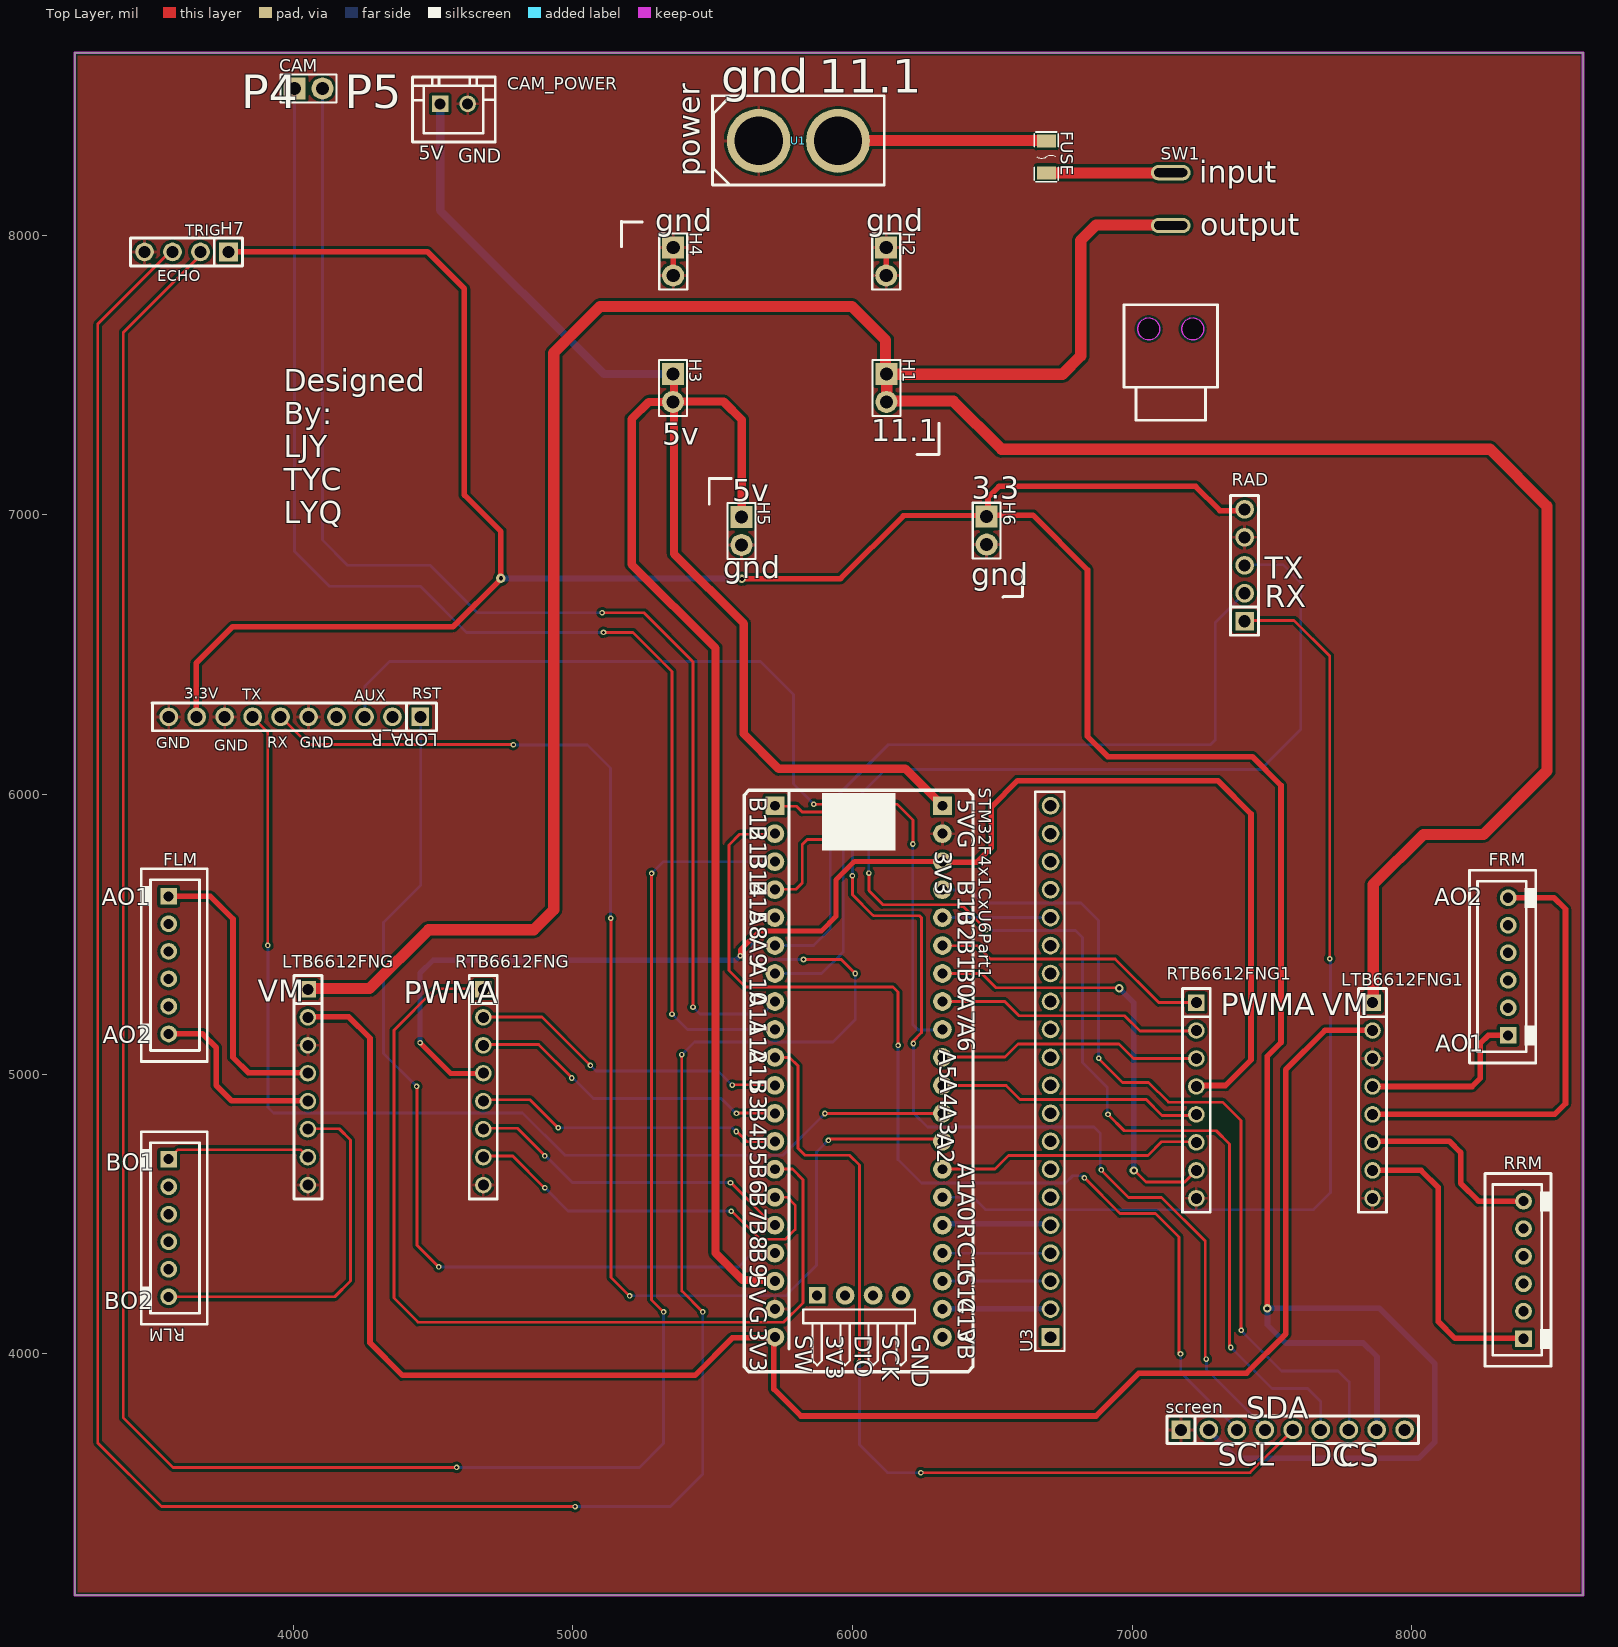
[diagram p0: Top Layer view]
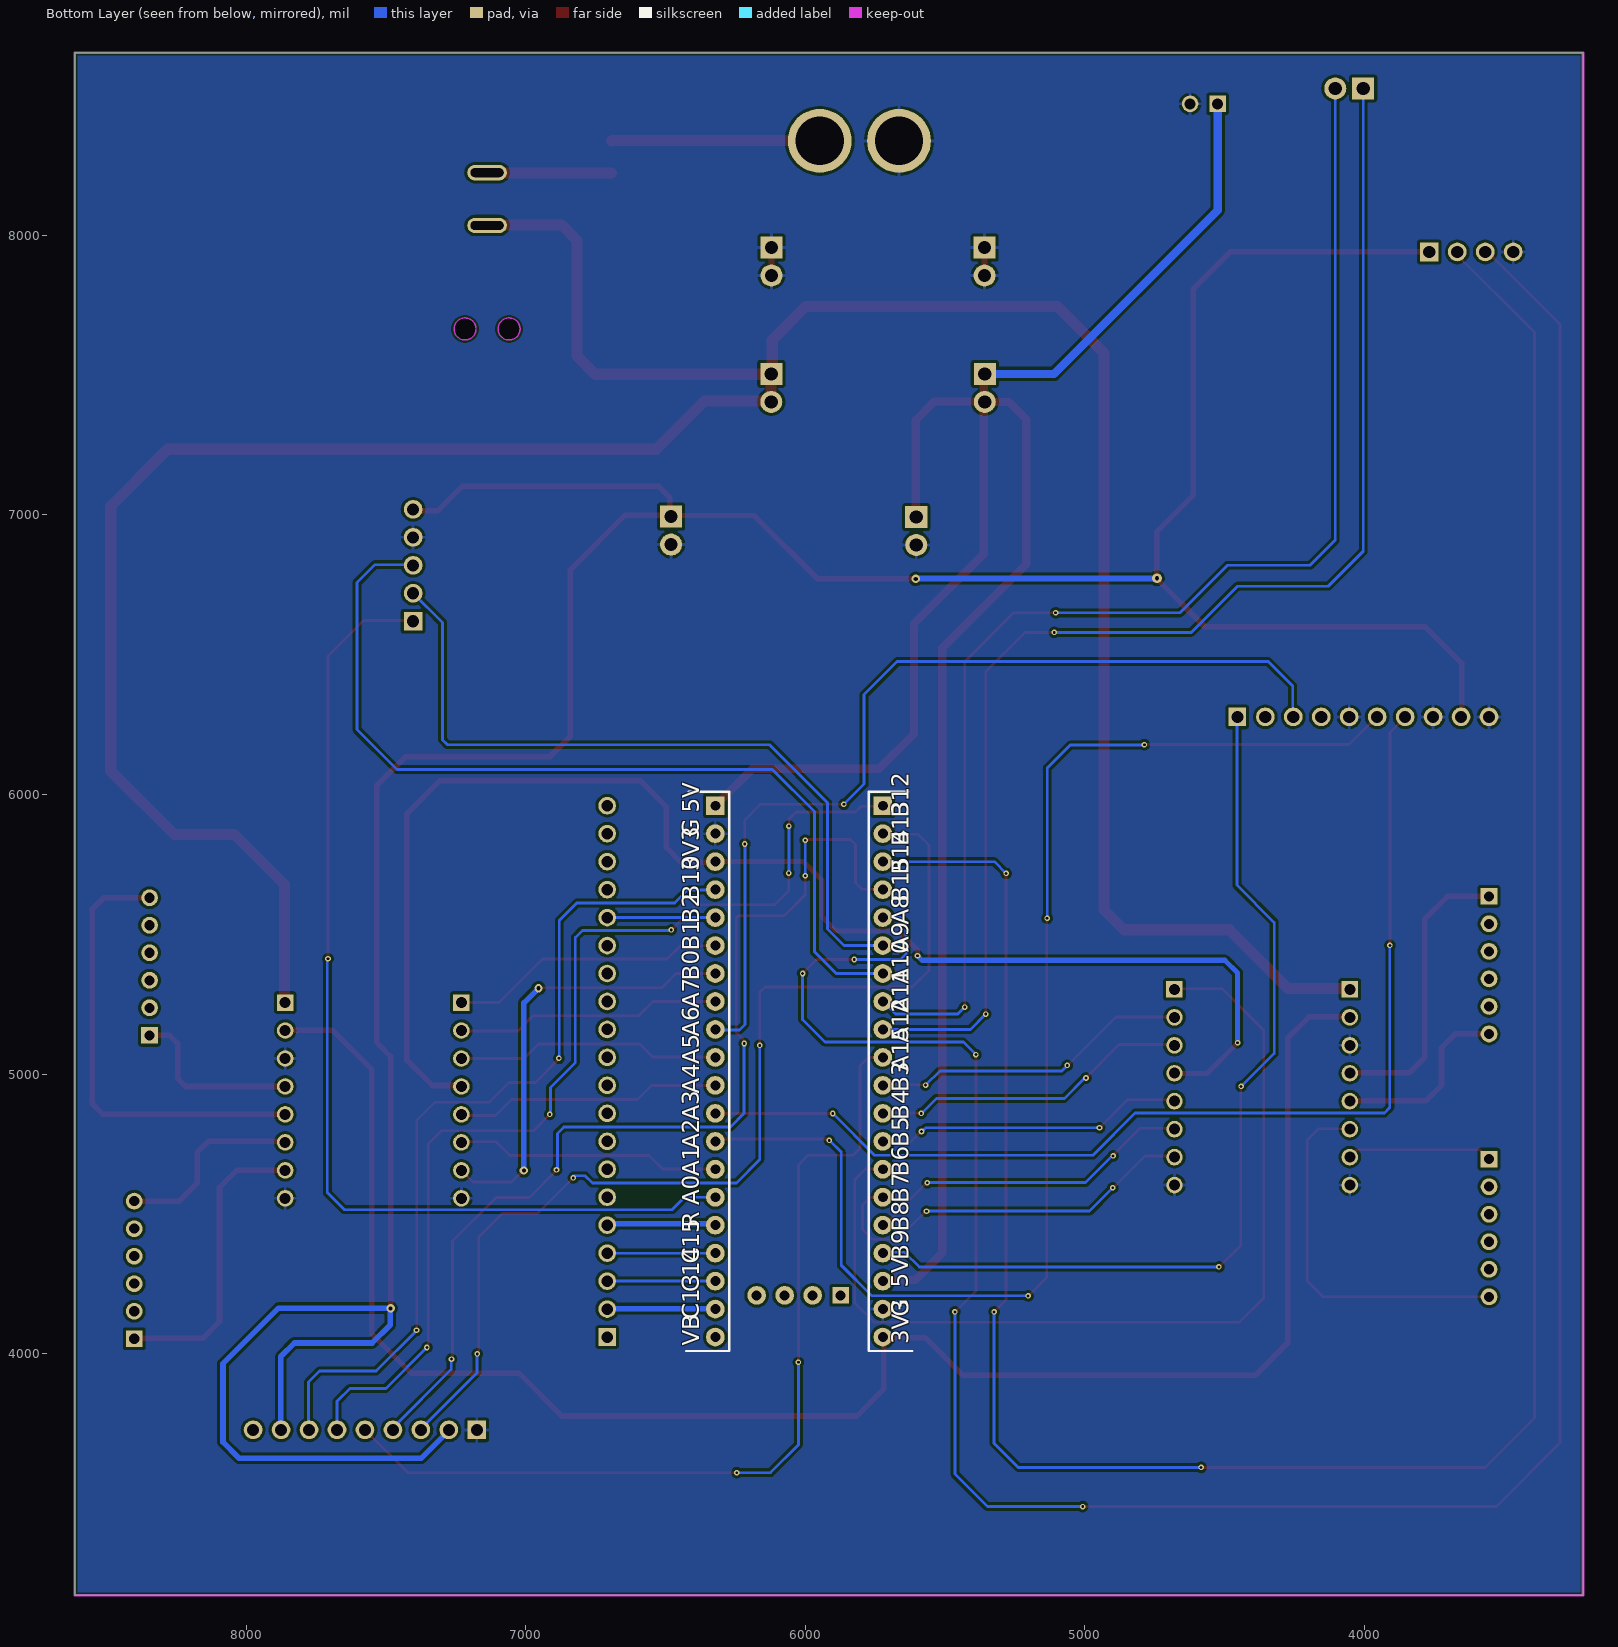
[diagram p1: Bottom Layer view, seen from below]
# Altium PCB MISC51978.pcbdoc
Units mil, origin at the board's own origin, x right, y up, seen from the top; angles counter-clockwise.
Board outline 5393.7 x 5516.21 mil, 2 copper layers (Top Layer, Bottom Layer), stack 62.206 mil thick; 25 components, 49 nets, 170 pads, 57 vias.

## Layer stack, top to bottom
Top Solder Mask Layer: solder mask 0.394, Dk 3.3
Top Layer: signal copper 1.379
Dielectric1: surface 59.449, FR4, Dk 4.5
Bottom Layer: signal copper 1.378
Bottom Solder Mask Layer: solder mask 0.394, Dk 3.3

## Board outline
3219.03,8652.78 3219.03,3136.57 8612.73,3136.57 8612.73,8652.78

## Design rules (kind name [scope] priority, off if disabled: settings)
BoardOutlineClearance copperThickness2oz_1 [All] p2 off: genericclearance=7.99 ignorepadtopadclearanceinfootprint=FALSE except(0: Arc-SplitContinuation Track-SplitContinuation SMDPad-SplitContinuation THPad-SplitContinuation Via-SplitContinuation Fill-SplitContinuation Region-SplitContinuation Poly-SplitContinuation Text-SplitContinuation Hole-SplitContinuation; 5.98: Arc-CutoutEdge SMDPad-CutoutEdge THPad-CutoutEdge Via-CutoutEdge Fill-CutoutEdge Region-CutoutEdge Text-CutoutEdge; 6.93: Hole-OutlineEdge Hole-CutoutEdge; 10: Poly-OutlineEdge Poly-CutoutEdge; 11.81: Arc-OutlineEdge Track-OutlineEdge SMDPad-OutlineEdge THPad-OutlineEdge Via-OutlineEdge Fill-OutlineEdge Region-OutlineEdge Text-OutlineEdge Track-CutoutEdge)
BoardOutlineClearance copperThickness1oz_1 [All] p4: genericclearance=6 ignorepadtopadclearanceinfootprint=FALSE except(0: Arc-SplitContinuation Track-SplitContinuation SMDPad-SplitContinuation THPad-SplitContinuation Via-SplitContinuation Fill-SplitContinuation Region-SplitContinuation Poly-SplitContinuation Text-SplitContinuation Hole-SplitContinuation; 6: Arc-CutoutEdge Track-CutoutEdge SMDPad-CutoutEdge THPad-CutoutEdge Via-CutoutEdge Text-CutoutEdge; 6.93: Hole-OutlineEdge Hole-CutoutEdge; 10: Poly-OutlineEdge Poly-CutoutEdge; 11.8: Arc-OutlineEdge Track-OutlineEdge SMDPad-OutlineEdge THPad-OutlineEdge Via-OutlineEdge Fill-OutlineEdge Region-OutlineEdge Text-OutlineEdge Fill-CutoutEdge Region-CutoutEdge)
Clearance copperThickness2oz [All] p1 off: gap=7.99 ignorepadtopadclearanceinfootprint=FALSE except(5.98: SMDPad-Track SMDPad-SMDPad THPad-Track SMDPad-THPad THPad-THPad Track-Via SMDPad-Via THPad-Via Via-Via Fill-Track Region-Track Fill-SMDPad Region-SMDPad Fill-THPad Region-THPad Fill-Via Region-Via Fill-Fill Fill-Region Region-Region Arc-Track Arc-SMDPad Arc-THPad Arc-Via Fill-Arc Region-Arc Arc-Arc Text-Track SMDPad-Text Text-THPad Text-Via Fill-Text Region-Text Arc-Text Text-Text; 6.93: Hole-Track Hole-SMDPad Hole-THPad Hole-Via Fill-Hole Region-Hole Hole-Arc Hole-Text; 10: Poly-Track Poly-SMDPad Poly-THPad Poly-Via Poly-Fill Poly-Region Poly-Poly Poly-Arc Poly-Text Poly-Hole)
Clearance copperThickness1oz [All] p3: gap=6 ignorepadtopadclearanceinfootprint=FALSE except(5.98: SMDPad-Track SMDPad-SMDPad THPad-Track SMDPad-THPad THPad-THPad Track-Via SMDPad-Via THPad-Via Via-Via Fill-SMDPad Region-SMDPad Fill-THPad Region-THPad Fill-Via Region-Via Fill-Fill Fill-Region Region-Region; 6.93: Hole-Track Hole-SMDPad Hole-THPad Hole-Via Fill-Hole Region-Hole Hole-Arc Hole-Text; 10: Poly-Track Poly-SMDPad Poly-THPad Poly-Via Poly-Fill Poly-Region Poly-Poly Poly-Arc Poly-Text Poly-Hole; 11.8: Fill-Track Region-Track)
DiffPairsRouting differentialPair [All] p1: maxlimit=6 minlimit=6 mostfreqgap=6 toplayer_minwidth=5 toplayer_prefwidth=10 toplayer_maxwidth=100 toplayer_mingap=6 toplayer_prefgap=6 toplayer_maxgap=6 bottomlayer_minwidth=5 bottomlayer_prefwidth=10 bottomlayer_maxwidth=100 bottomlayer_mingap=6 bottomlayer_prefgap=6 bottomlayer_maxgap=6 maxuncoupledlength=10
HoleToHoleClearance otherClearance [All] p1: gap=11.81 allowstackedmicrovias=TRUE
Length netLength [All] p1: minlimit=0 maxlimit=0
MatchedLengths netLengthTolerance [All] p1: tolerance=1000
PasteMaskExpansion pasteMaskExpansion [All] p1: expansion=0
PlaneConnect innerPlane [All] p1: planeconnectstyle=Relief reliefexpansion=20 reliefentries=4 reliefconductorwidth=10 reliefairgap=10
PolygonConnect "copperRegion_Top Layer" [(InNet('GND')) And OnLayer('Top Layer')] p1: connectstyle=Relief reliefconductorwidth=10 reliefentries=4 polygonreliefangle="90 Angle" airgapwidth=10 via.connectstyle=Relief via.reliefconductorwidth=10 via.reliefentries=4 via.polygonreliefangle="90 Angle" via.airgapwidth=10
PolygonConnect "copperRegion_Bottom Layer" [(InNet('GND')) And OnLayer('Bottom Layer')] p2: connectstyle=Relief reliefconductorwidth=10 reliefentries=4 polygonreliefangle="90 Angle" airgapwidth=10 via.connectstyle=Relief via.reliefconductorwidth=10 via.reliefentries=4 via.polygonreliefangle="90 Angle" via.airgapwidth=10
PolygonConnect copperRegion [(InNet('GND'))] p3: connectstyle=Direct reliefconductorwidth=10 reliefentries=4 polygonreliefangle="90 Angle" airgapwidth=10 via.connectstyle=Relief via.reliefconductorwidth=10 via.reliefentries=4 via.polygonreliefangle="90 Angle" via.airgapwidth=10
RoutingVias viaSize [All] p1: holewidth=10 width=20 viastyle="Through Hole" minholewidth=9 minwidth=19.68 maxholewidth=248.03 maxwidth=393.7
SolderMaskExpansion solderMaskExpansion [IsVia] p1: expansion=-1000 istentingtop=TRUE
SolderMaskExpansion solderMaskExpansion [All] p2: expansion=2 istentingtop=FALSE
Width copperThickness2oz_2 [All] p1 off: maxlimit=100 minlimit=8 preferedwidth=10
Width copperThickness1oz_2 [All] p2: maxlimit=10 minlimit=10 preferedwidth=10 toplayer_minwidth=5 toplayer_maxwidth=100 toplayer_prefwidth=10 bottomlayer_minwidth=5 bottomlayer_maxwidth=100 bottomlayer_prefwidth=10

## Components (designator, comment, footprint, x,y, rotation, side; value= is the part's Value field where it differs from the comment)
CAM "PZ254V-11-02P" HDR-TH_2P-P2.54-V-M 4055,8525 r0 top
CAM_POWER "HX-XH2.54-2PZZ" CONN-TH_2P-P2.50_HX-2.54MM-2P-ZZ-MS 4575,8470 r0 top
FLM "HX-XH2.54-6PZZ" CONN-TH_6P-P2.50_BX-XH2.54-6PZZ 3555,5390 r270 top
FRM "HX-XH2.54-6PZZ" CONN-TH_6P-P2.50_BX-XH2.54-6PZZ 8345,5385 r90 top
FUSE "" F1206 6693.35,8280.21 r270 top
H1 "PZ254V-11-02P" HDR-TH_2P-P2.54-V-M 6121.83,7454.08 r270 top
H2 "PZ254V-11-02P" HDR-TH_2P-P2.54-V-M 6120.91,7906.02 r270 top
H3 "PZ254V-11-02P" HDR-TH_2P-P2.54-V-M 5358.22,7454 r270 top
H4 "PZ254V-11-02P" HDR-TH_2P-P2.54-V-M 5359.02,7905.96 r270 top
H5 "PZ254V-11-02P" HDR-TH_2P-P2.54-V-M 5603.37,6942.34 r270 top
H6 "PZ254V-11-02P" HDR-TH_2P-P2.54-V-M 6480.05,6943.82 r270 top
H7 "PZ254V-11-04P" HDR-TH_4P-P2.54-V-M 3618.69,7940.45 r180 top
LORA_R "PZ254V-11-10P" HDR-TH_10P-P2.54-V-M 4005.16,6277.81 r180 top
LTB6612FNG "PZ254V-11-08P" HDR-TH_8P-P2.54-V-M 4052.95,4953.4 r270 top
LTB6612FNG1 "PZ254V-11-08P" HDR-TH_8P-P2.54-V-M 7860.02,4906.07 r270 top
RAD "PZ254V-11-05P" HDR-TH_5P-P2.54-V-M 7402.6,6819.77 r90 top
RLM "HX-XH2.54-6PZZ" CONN-TH_6P-P2.50_BX-XH2.54-6PZZ 3555,4450 r270 top
RRM "HX-XH2.54-6PZZ" CONN-TH_6P-P2.50_BX-XH2.54-6PZZ 8400,4300 r90 top
RTB6612FNG "PZ254V-11-08P" HDR-TH_8P-P2.54-V-M 4680.06,4953.4 r270 top
RTB6612FNG1 "PZ254V-11-08P" HDR-TH_8P-P2.54-V-M 7230.02,4906.07 r270 top
screen "PZ254V-11-09P" HDR-TH_9P-P2.54-V-M 7574.85,3728.09 r0 top
STM32F4x1CxU6Part1 "STM32F4x1CxU6 WeActStudio" "STM32F4x1CxU6 WeActStudio" 5975,5245 r270 top
SW1 "HX KCD11-BL" SW-TH_KCD11-BL 7138.26,8129.56 r0 top
U1 "XT60-M." CONN-TH_XT60 5806.73,8337.63 r0 top
U3 "ZX-PZ2.54-1-20PZZ" HDR-TH_20P-P2.54-V-M 6708.51,5010 r90 top

## Footprints (in the part's own frame and the unit in brackets; to place one, negate y for a bottom-side part, rotate by r counter-clockwise, add the part's x,y. Pads: shape width x height; smd on the part's side, far side on the other; paste and mask are expansions set on the pad)
CONN-TH_2P-P2.50_HX-2.54MM-2P-ZZ-MS [mm]
  rect 1.5x1.5 hole 1: 1(-1.25,0)
  round 1.5 hole 1: 2(1.25,0)
  silkscreen extent -3.75,-3.46 3.75,2.44
CONN-TH_6P-P2.50_BX-XH2.54-6PZZ [mil]
  rect 60x60 hole 36: 1(-246.07,0)
  round 60 hole 36: 2(-147.65,0) 3(-49.22,0) 4(49.2,0) 5(147.63,0) 6(246.06,0)
  silkscreen extent -344,-100 344,138
CONN-TH_XT60 [mm]
  round 5.8 hole 4.4 paste+0 mask+0.05: 1(-3.6,0) 2(3.6,0)
  silkscreen extent -7.8,-4 7.8,4.1
F1206 [mm]
  rect 1.19x1.728 smd: 1(-1.445,0) 2(1.445,0)
  silkscreen extent -2.27,-1.09 2.27,1.09
HDR-TH_2P-P2.54-V-M [mm]
  rect 2x2 hole 1.2: 1(-1.27,0)
  round 2 hole 1.2: 2(1.27,0)
  silkscreen extent -2.54,-1.27 2.54,1.27
HDR-TH_4P-P2.54-V-M [mm]
  rect 1.7x1.7 hole 1.1: 1(-3.81,0)
  round 1.7 hole 1.1: 2(-1.27,0) 3(1.27,0) 4(3.81,0)
  silkscreen extent -5.08,-1.27 5.08,1.27
HDR-TH_5P-P2.54-V-M [mm]
  rect 1.7x1.7 hole 1.1: 1(-5.08,0)
  round 1.7 hole 1.1: 2(-2.54,0) 3(0,0) 4(2.54,0) 5(5.08,0)
  silkscreen extent -6.35,-1.27 6.35,1.27
HDR-TH_8P-P2.54-V-M [mm]
  rect 1.5x1.5 hole 1: 1(-8.89,0)
  round 1.5 hole 1: 2(-6.35,0) 3(-3.81,0) 4(-1.27,0) 5(1.27,0) 6(3.81,0) 7(6.35,0) 8(8.89,0)
  silkscreen extent -10.16,-1.27 10.16,1.27
HDR-TH_9P-P2.54-V-M [mm]
  rect 1.7x1.7 hole 1.1: 1(-10.16,0)
  round 1.7 hole 1.1: 2(-7.62,0) 3(-5.08,0) 4(-2.54,0) 5(0,0) 6(2.54,0) 7(5.08,0) 8(7.62,0) 9(10.16,0)
  silkscreen extent -11.43,-1.25 11.43,1.25
HDR-TH_10P-P2.54-V-M [mm]
  rect 1.575x1.7 hole 1.1: 1(-11.43,0)
  round 1.7 hole 1.1: 2(-8.89,0) 3(-6.35,0) 4(-3.81,0) 5(-1.27,0) 6(1.27,0) 7(3.81,0) 8(6.35,0) 9(8.89,0) 10(11.43,0)
  silkscreen extent -12.9,-1.27 12.95,1.27
HDR-TH_20P-P2.54-V-M [mm]
  rect 1.6x1.6 hole 1.05: 1(-24.13,0)
  round 1.6 hole 1.05: 2(-21.59,0) 3(-19.05,0) 4(-16.51,0) 5(-13.97,0) 6(-11.43,0) 7(-8.89,0) 8(-6.35,0) 9(-3.81,0) 10(-1.27,0) 11(1.27,0) 12(3.81,0) 13(6.35,0) 14(8.89,0) 15(11.43,0) 16(13.97,0) 17(16.51,0) 18(19.05,0) 19(21.59,0) 20(24.13,0)
  silkscreen extent -25.4,-1.27 25.4,1.4
"STM32F4x1CxU6 WeActStudio" [mm]
  rect 1.7x1.7 hole 0.9: 1(-18.161,-6.401) 40(-18.161,8.814)
  round 1.7 hole 0.9: 2(-15.621,-6.401) 3(-13.081,-6.401) 4(-10.541,-6.401) 5(-8.001,-6.401) 6(-5.461,-6.401) 7(-2.921,-6.401) 8(-0.381,-6.401) 9(2.159,-6.401) 10(4.699,-6.401) 11(7.239,-6.401) 12(9.779,-6.401) 13(12.319,-6.401) 14(14.859,-6.401) 15(17.399,-6.401) 16(19.939,-6.401) 17(22.479,-6.401) 18(25.019,-6.401) 19(27.559,-6.401) 20(30.099,-6.401) 21(30.099,8.814) 22(27.559,8.814) 23(25.019,8.814) 24(22.479,8.814) 25(19.939,8.814) 26(17.399,8.814) 27(14.859,8.814) 28(12.319,8.814) 29(9.779,8.814) 30(7.239,8.814) 31(4.699,8.814) 32(2.159,8.814) 33(-0.381,8.814) 34(-2.921,8.814) 35(-5.461,8.814) 36(-8.001,8.814) 37(-10.541,8.814) 38(-13.081,8.814) 39(-15.621,8.814) 42(26.314,-0.025) 43(26.314,2.515) 44(26.314,5.055)
  rect 1.5x1.5 hole 0.9: 41(26.314,-2.565)
  silkscreen extent -19.56,-9.19 33.25,11.58
SW-TH_KCD11-BL [mm]
  oval 3.6x1.4 hole 0.8 slot 3 at 0 deg paste+0 mask+0.05: 1(0,2.4) 2(0,-2.4)
  Board Outline Layer circle w0.003: c-2,-11.8 r1
  Board Outline Layer circle w0.003: c2,-11.8 r1
  Board Outline Layer region: -1,-11.8 -1.099,-12.234 -1.377,-12.582 -1.777,-12.775 -2.223,-12.775 -2.623,-12.582 -2.901,-12.234 -3,-11.8 -3,-11.8 -2.901,-11.366 -2.623,-11.018 -2.223,-10.825 -1.777,-10.825 -1.377,-11.018 -1.099,-11.366 -1,-11.8
  Board Outline Layer region: -1,-11.8 -1.009,-11.936 -1.037,-12.07 -1.083,-12.198 -1.146,-12.319 -1.224,-12.431 -1.317,-12.531 -1.423,-12.617 -1.54,-12.688 -1.665,-12.742 -1.797,-12.779 -1.932,-12.798 -2.068,-12.798 -2.203,-12.779 -2.335,-12.742 -2.46,-12.688 -2.577,-12.617 -2.683,-12.531 -2.776,-12.431 -2.854,-12.319 -2.917,-12.198 -2.963,-12.07 -2.991,-11.936 -3,-11.8 -2.991,-11.664 -2.963,-11.53 -2.917,-11.401 -2.854,-11.28 -2.776,-11.169 -2.683,-11.069 -2.577,-10.983 -2.46,-10.912 -2.335,-10.858 -2.203,-10.821 -2.068,-10.802 -1.932,-10.802 -1.797,-10.821 -1.665,-10.858 -1.54,-10.912 -1.423,-10.983 -1.317,-11.069 -1.224,-11.169 -1.146,-11.28 -1.083,-11.401 -1.037,-11.53 -1.009,-11.664
  Board Outline Layer region: 3,-11.8 2.901,-12.234 2.623,-12.582 2.223,-12.775 1.777,-12.775 1.377,-12.582 1.099,-12.234 1,-11.8 1,-11.8 1.099,-11.366 1.377,-11.018 1.777,-10.825 2.223,-10.825 2.623,-11.018 2.901,-11.366 3,-11.8
  Board Outline Layer region: 3,-11.8 2.991,-11.936 2.963,-12.07 2.917,-12.198 2.854,-12.319 2.776,-12.431 2.683,-12.531 2.577,-12.617 2.46,-12.688 2.335,-12.742 2.203,-12.779 2.068,-12.798 1.932,-12.798 1.797,-12.779 1.665,-12.742 1.54,-12.688 1.423,-12.617 1.317,-12.531 1.224,-12.431 1.146,-12.319 1.083,-12.198 1.037,-12.07 1.009,-11.936 1,-11.8 1.009,-11.664 1.037,-11.53 1.083,-11.401 1.146,-11.28 1.224,-11.169 1.317,-11.069 1.423,-10.983 1.54,-10.912 1.665,-10.858 1.797,-10.821 1.932,-10.802 2.068,-10.802 2.203,-10.821 2.335,-10.858 2.46,-10.912 2.577,-10.983 2.683,-11.069 2.776,-11.169 2.854,-11.28 2.917,-11.401 2.963,-11.53 2.991,-11.664
  Multi-Layer board cut-out: -1,-11.8 -1.099,-12.234 -1.377,-12.582 -1.777,-12.775 -2.223,-12.775 -2.623,-12.582 -2.901,-12.234 -3,-11.8 -3,-11.8 -2.901,-11.366 -2.623,-11.018 -2.223,-10.825 -1.777,-10.825 -1.377,-11.018 -1.099,-11.366 -1,-11.8
  Multi-Layer board cut-out: 3,-11.8 2.901,-12.234 2.623,-12.582 2.223,-12.775 1.777,-12.775 1.377,-12.582 1.099,-12.234 1,-11.8 1,-11.8 1.099,-11.366 1.377,-11.018 1.777,-10.825 2.223,-10.825 2.623,-11.018 2.901,-11.366 3,-11.8
  silkscreen extent -4.25,-20.1 4.25,-9.6

## Via types
v1: diameter 20, hole 10, Top Layer to Bottom Layer, 52 vias
v2: diameter 30, hole 15, Top Layer to Bottom Layer, 4 vias
v3: diameter 35, hole 15, Top Layer to Bottom Layer, 1 vias

## Nets (pads, with @x,y where several pads share a name; then routed paths per layer and width w, separated by ;. In a path a pad name is that pad's centre, name@x,y a point inside that pad or via, vN(x,y) a via of type N, cw(c..) or ccw(c..) an arc to the next point about the centre after c; other vN are vias at no path point)
CAM_P4: CAM.1 STM32F4x1CxU6Part1.9 | length 4798.9
  Top Layer w10: v1(5110,6580) 5215,6580 5355,6440 v1(5355,5215)
  Bottom Layer w10: CAM.1 4005,6870 4130,6745 4455,6745 4620,6580 v1(5110,6580) ; v1(5355,5215) 5410,5160 STM32F4x1CxU6Part1.9
CAM_P5: CAM.2 STM32F4x1CxU6Part1.8 | length 4677.2
  Top Layer w10: v1(5105,6650) 5255,6650 5430,6475 v1(5430,5240)
  Bottom Layer w10: CAM.2 4105,6910 4195,6820 4490,6820 4660,6650 v1(5105,6650) ; v1(5430,5240) 5455,5215 5678,5215 STM32F4x1CxU6Part1.8
GND: CAM_POWER.2 H2.1 H2.2 H4.1 H4.2 H5.2 H6.2 H7.4 LORA_R.5 LORA_R.8 LORA_R.10 LTB6612FNG1.3 LTB6612FNG1.8 LTB6612FNG.3 LTB6612FNG.8 RAD.4 RTB6612FNG1.8 RTB6612FNG.8 screen.1 STM32F4x1CxU6Part1.19 STM32F4x1CxU6Part1.39 U1.1 | length 201.1
  Top Layer w20: H4.2@5359.4,7854.66 H4.1@5359.4,7955.86 ; H2.2@6121.01,7857.25 H2.1@6121.01,7957.15
HC_ECHO: H7.3 STM32F4x1CxU6Part1.5 | length 9646.4
  Top Layer w10: H7.3@3563.74,7944.74 3301,7682.01 3301,3681.84 3529.03,3453.82 v1(5008.21,3453.82) ; v1(5390,5070) 5390,4225 v1(5465,4150) ; v1(5825,5410) 5960,5410 v1(6010,5360)
  Bottom Layer w10: v1(5008.21,3453.82) 5348.82,3453.82 5465,3570 v1(5465,4150) ; v1(5390,5070) 5435,5115 5930,5115 6010,5195 v1(6010,5360) ; STM32F4x1CxU6Part1.5 5660,5560 5640,5540 5640,5430 5660,5410 v1(5825,5410)
HC_TRIG: H7.2 STM32F4x1CxU6Part1.3 | length 8841.6
  Top Layer w10: H7.2@3678.57,7938.78 3392.84,7653.06 3392.84,3771.13 3570.11,3593.86 v1(4584.69,3593.86) ; v1(5281.96,5718.04) 5281.96,4193.04 v1(5325,4150)
  Bottom Layer w10: v1(4584.69,3593.86) 5238.86,3593.86 5325,3680 v1(5325,4150) ; v1(5281.96,5718.04) 5323.93,5760 STM32F4x1CxU6Part1.3
L_AIN1: RTB6612FNG.3 STM32F4x1CxU6Part1.12 | length 1136
  Top Layer w10: RTB6612FNG.3@4685.41,5105.65 4878.08,5105.65 v1@4994.85,4988.88 ; v1@5585.63,4861.57 5720.56,4861.57 STM32F4x1CxU6Part1.12@5724.89,4857.24
  Bottom Layer w10: v1@4997.44,4986.13 5000.9,4986.13 5073.56,4913.47 5531.13,4913.47 v1@5583.03,4861.57
  other v1: 5585.63,4859.84 4996.5,4986.28
L_AIN2: RTB6612FNG.2 STM32F4x1CxU6Part1.11 | length 1142.5
  Top Layer w10: RTB6612FNG.2@4676.65,5204.9 4889.46,5204.9 v1(5063.1,5031.26) ; v1@5570.92,4961.91 5720.56,4961.91 STM32F4x1CxU6Part1.11@5721.43,4961.04
  Bottom Layer w10: v1(5063.1,5031.26) 5082.88,5011.48 5518.97,5011.48 v1@5567.89,4962.56
  other v1: 5570.06,4961.04
L_AO1: FLM.1 LTB6612FNG.4 | length 1050
  Top Layer w20: FLM.1 3703.93,5636.06 3785,5555 3785,5060 3840,5005 4051.34,5005 LTB6612FNG.4
L_AO2: FLM.6 LTB6612FNG.5 | length 676.7
  Top Layer w20: FLM.6 3676.07,5143.94 3725,5095 3725,4960 3780,4905 4051.34,4905 LTB6612FNG.5
L_BIN1: RTB6612FNG.5 STM32F4x1CxU6Part1.13 | length 1096.1
  Top Layer w10: RTB6612FNG.5@4683.38,4908.76 4847.4,4908.76 v1(4948.06,4808.1) ; v1@5586.49,4794.97 5622.82,4758.64 STM32F4x1CxU6Part1.13@5721.43,4758.64
  Bottom Layer w10: v1(4948.06,4808.1) 4948.77,4808.81 5569.19,4808.81 v1@5582.17,4795.83
  other v1: 5584.76,4794.97
L_BIN2: RTB6612FNG.6 STM32F4x1CxU6Part1.16 | length 1169.6
  Top Layer w10: RTB6612FNG.6@4686.3,4806.58 4803.07,4806.58 v1@4899.41,4710.25 ; v1@5566.6,4610.73 5719.7,4457.63 STM32F4x1CxU6Part1.16@5722.29,4457.63
  Bottom Layer w10: v1@4901.43,4709.33 4998.31,4612.46 v1@5558.81,4612.46
  other v1: 5564,4611.59 4899.62,4707.76
L_BO1: LTB6612FNG.7 RLM.1 | length 523
  Top Layer w10: RLM.1 3588.93,4730 4026.34,4730 LTB6612FNG.7
L_BO2: LTB6612FNG.6 RLM.6 | length 1347.5
  Top Layer w10: RLM.6 4148.94,4203.94 4205,4260 4205,4765 4165,4805 4054.55,4805 LTB6612FNG.6
L_PWMA: RTB6612FNG.1 STM32F4x1CxU6Part1.14 | length 3417
  Top Layer w10: RTB6612FNG.1@4681.84,5305.78 4509.6,5305.78 4360.71,5156.9 4360.71,4199.37 4446.94,4113.15 5754.57,4113.15 5823.28,4181.85 5823.28,4622.67 5785.33,4660.62 STM32F4x1CxU6Part1.14@5729.86,4660.62
L_PWMB: RTB6612FNG.7 STM32F4x1CxU6Part1.15 | length 1410.4
  Top Layer w10: RTB6612FNG.7@4686.3,4707.33 4785.55,4707.33 v1@4899.41,4593.47 ; v1@5570.06,4509.52 5669.53,4410.05 5761.22,4410.05 5795.38,4444.22 5795.38,4531.58 5767.27,4559.69 STM32F4x1CxU6Part1.15@5725.75,4559.69
  Bottom Layer w10: v1@4899.7,4594.29 4983.6,4510.39 v1@5565.73,4510.39
  other v1: 5566.6,4509.52 4900.49,4593.58
LORA_AUX: LORA_R.3 STM32F4x1CxU6Part1.32 | length 3357.7
  Top Layer w10: v1@5864.14,5965.65 6159.96,5965.65 6216.4,5909.21 v1@6216.4,5823.57
  Bottom Layer w10: LORA_R.3@4257.2,6287.4 4257.2,6388.11 4344.78,6475.69 5671.6,6475.69 5789.83,6357.46 5789.83,6037.8 v1@5859.89,5967.74 ; v1@6215.88,5823.72 6215.88,5177.58 6235.34,5158.12 6317.08,5158.12 STM32F4x1CxU6Part1.32@6319.67,5160.71
  other v1: 6216.4,5823.24 5862.1,5965.14
LORA_RST: LORA_R.1 STM32F4x1CxU6Part1.17 | length 3330.7
  Top Layer w10: v1@4442.72,4957.37 4442.72,4388.26 v1@4520.57,4310.41
  Bottom Layer w10: v1@4441.94,4955.84 4323.51,5074.27 4323.51,5543.04 4456.74,5676.27 LORA_R.1@4456.74,6278.27 ; v1@4521.55,4310.29 5592.31,4310.29 5644.95,4362.92 5722.25,4362.92 STM32F4x1CxU6Part1.17@5723.9,4361.28
  other v1: 4520.94,4310.9 4441.62,4956.27
LORA_RX: LORA_R.6 STM32F4x1CxU6Part1.28 | length 4743.9
  Top Layer w10: LORA_R.6@3956.64,6277.74 4055.6,6178.78 v1@4787.81,6178.78 ; v1@5136.53,5557.82 5136.53,4273.22 v1@5202.32,4207.43 ; v1@5917.14,4768.52 6311.89,4768.52 STM32F4x1CxU6Part1.28@6316.83,4763.59
  Bottom Layer w10: v1@4791.91,6176.68 5052.67,6176.68 5134.94,6094.41 ; v1@5134.94,5558.43 5134.94,6090.51 ; 5134.94,6094.63 5134.94,6094.41 ; v1@5205.24,4207.98 5762.83,4207.98 5871.39,4316.54 5871.39,4721.16 v1@5913.33,4763.1 ; 5134.94,6090.51 5135.13,6090.32 5134.94,6094.03 ; 5134.94,6090.51 5134.94,6094.03 ; 5134.94,6094.03 5134.94,6094.41
  other v1: 5203.42,4207.07 5914.22,4763.38 5135.61,5557.27 4787.63,6178.32
LORA_TX: LORA_R.7 STM32F4x1CxU6Part1.29 | length 3959.6
  Top Layer w10: LORA_R.7@3858.05,6273.73 3909.56,6222.22 v1(3909.56,5460.43) ; v1@5902.23,4859.72 6321.84,4859.72 STM32F4x1CxU6Part1.29@6322.82,4860.69
  Bottom Layer w10: v1(3909.56,5460.43) 3910,5459.98 3910,4880.72 3929.51,4861.2 4820.72,4861.2 4971.77,4710.16 5752.51,4710.16 v1@5901.63,4859.29
  other v1: 5901.75,4859.43
P2_11.1V: FUSE.2 SW1.1 | length 446.7
  Top Layer w40: FUSE.2@6694.06,8223.13 7139.52,8223.13 SW1.1@7140.38,8224
P_3.3V: H6.1 H7.1 LORA_R.9 RAD.5 screen.2 screen.8 | length 12534.8
  Top Layer w10: v3@4742.86,6771.33 v3@4744.8,6771.33
  Top Layer w20: LORA_R.9@3652.99,6280.89 3652.99,6469.67 3783.38,6600.06 4571.59,6600.06 v3@4742.86,6771.33 ; H7.1@3769.76,7940.99 4480.12,7940.99 4612.46,7808.65 4612.46,7071.15 4742.86,6940.76 v3@4742.86,6777.17 ; v2@5607.13,6772.03 5957.44,6772.03 6182.23,6996.82 H6.1@6478.89,6999.18 ; RAD.5@7402.73,7022.87 7395.33,7015.47 7313.91,7015.47 7227.56,7101.82 6524.4,7101.82 6484.93,7062.34 6484.93,6999.21 6645.29,6999.21 6840.88,6803.62 6840.88,6208.09 6913.86,6135.1 7430.58,6135.1 7532.75,6032.93 7532.75,5113.35 7483.12,5063.72 v2@7483.12,4164.58
  Bottom Layer w20: v3@4743.77,6772.6 v2@5603.99,6772.6 ; screen.2@7271.09,3729.38 7374.16,3626.31 8024.41,3626.31 8082.53,3684.43 8082.53,3965.14 7884.05,4163.61 7484.42,4163.61 7484.42,4103.4 7549.01,4038.81 7826.95,4038.81 7875.97,3989.8 7875.97,3730.3 screen.8@7874.82,3729.15
  other v2: 7483.3,4162.5 5604.98,6771.26
  other v3: 4742.88,6773.23
P_5V: CAM_POWER.1 H3.1 H3.2 H5.1 STM32F4x1CxU6Part1.18 STM32F4x1CxU6Part1.40 | length 7796.5
  Top Layer w20: H3.1@5359.72,7505.09 H3.1@5360.79,7505.09
  Top Layer w30: H3.2@5357.13,7403.74 5271.82,7403.74 5210.62,7342.55 5210.62,6823.34 5510.39,6523.58 5510.39,4360.38 5606.73,4264.04 STM32F4x1CxU6Part1.18@5724.96,4264.04 ; H3.1@5359.72,7505.09 H3.1@5359.72,7505.32 ; H3.2@5362.03,7403.74 5362.03,6860.74 5611.63,6611.14 5611.63,6217.04 5736.43,6092.24 6189.65,6092.24 STM32F4x1CxU6Part1.40@6314.45,5967.44 ; H3.2@5362.03,7409.95 H3.1@5362.03,7505.09 ; H3.2@5363.28,7406.97 5540.07,7404.76 5604.94,7339.89 H5.1@5604.94,6993
  Bottom Layer w30: CAM_POWER.1 4525.78,8089.22 5111,7504 H3.1
P_11.1V: FUSE.1 U1.2 | length 744.2
  Top Layer w40: U1.2@5949.91,8338.81 6691.72,8338.81 FUSE.1
PB2: STM32F4x1CxU6Part1.36 U3.16 | length 386.5
  Bottom Layer w10: STM32F4x1CxU6Part1.36 U3.16
PC13: STM32F4x1CxU6Part1.22 U3.2 | length 385.3
  Bottom Layer w20: STM32F4x1CxU6Part1.22@6323.41,4161.87 U3.2@6708.76,4161.87
PC14: STM32F4x1CxU6Part1.23 U3.3 | length 386.5
  Bottom Layer w10: STM32F4x1CxU6Part1.23 U3.3
PC15: STM32F4x1CxU6Part1.24 U3.4 | length 386.5
  Bottom Layer w10: STM32F4x1CxU6Part1.24 U3.4
POWER_11.1V: H1.1 H1.2 LTB6612FNG1.1 LTB6612FNG.1 SW1.2 | length 10649.8
  Top Layer w40: LTB6612FNG.1@4054.52,5306.14 4273.46,5306.14 4483.65,5516.33 4860.24,5516.33 4931.76,5587.85 4931.76,7578.81 5098.16,7745.21 5998.76,7745.21 6118.46,7625.52 H1.1@6118.46,7507.28 ; H1.2@6115.17,7407.51 6360.39,7407.51 6532.91,7235 8280,7235 8484.18,7030.82 8484.18,6085.07 8256.47,5857.37 8041.9,5857.37 7862.37,5677.83 LTB6612FNG1.1@7862.37,5270.59 ; H1.2@6122.96,7408.23 H1.1@6122.96,7501.98 ; H1.1@6123.61,7503.04 6751.58,7503.04 6816.45,7567.92 6816.45,7981.81 6870.94,8036.3 SW1.2@7139.52,8036.3
R_AIN1: RTB6612FNG1.3 STM32F4x1CxU6Part1.31 | length 945.1
  Top Layer w10: STM32F4x1CxU6Part1.31@6324.09,5060.93 6545.52,5060.93 6592.23,5107.64 6953.79,5107.64 7005.69,5055.74 7227.12,5055.74 RTB6612FNG1.3@7227.99,5056.61
R_AIN2: RTB6612FNG1.2 STM32F4x1CxU6Part1.33 | length 950.8
  Top Layer w10: STM32F4x1CxU6Part1.33@6323.23,5259.87 6544.66,5259.87 6595.69,5208.84 6973.69,5208.84 7028.18,5154.35 7225.39,5154.35 RTB6612FNG1.2@7228.85,5157.81
R_AO1: FRM.1 LTB6612FNG1.4 | length 634
  Top Layer w20: LTB6612FNG1.4 8216.07,4956.07 8245,4985 8245,5110 8273.93,5138.94 FRM.1
R_AO2: FRM.6 LTB6612FNG1.5 | length 1623.1
  Top Layer w20: LTB6612FNG1.5 8511.07,4856.07 8550,4895 8550,5590 8508.93,5631.06 FRM.6
R_BIN1: RTB6612FNG1.5 STM32F4x1CxU6Part1.30 | length 953.4
  Top Layer w10: STM32F4x1CxU6Part1.30@6322.36,4959.73 6549.85,4959.73 6600.02,4909.56 7050.67,4909.56 7107.76,4852.47 7228.85,4852.47 RTB6612FNG1.5@7230.58,4854.2
R_BIN2: RTB6612FNG1.6 STM32F4x1CxU6Part1.27 | length 953.7
  Top Layer w10: STM32F4x1CxU6Part1.27@6323.23,4660.88 6510.06,4660.88 6558.5,4709.32 7056.72,4709.32 7105.6,4758.19 RTB6612FNG1.6@7236.64,4758.19
R_BO1: LTB6612FNG1.7 RRM.1 | length 1070.6
  Top Layer w20: LTB6612FNG1.7 8033.93,4656.07 8095,4595 8095,4115 8155,4055 8398.93,4055 RRM.1
R_BO2: LTB6612FNG1.6 RRM.6 | length 694.7
  Top Layer w20: LTB6612FNG1.6 7863.94,4760 8135,4760 8175,4720 8175,4610 8238.93,4546.06 RRM.6
R_PWMA: RTB6612FNG1.1 STM32F4x1CxU6Part1.35 | length 992.9
  Top Layer w10: STM32F4x1CxU6Part1.35@6322.14,5459.03 6447.57,5459.03 6494.27,5412.33 6939.74,5412.33 7095.43,5256.63 RTB6612FNG1.1@7231.23,5256.63
R_PWMB: RTB6612FNG1.7 STM32F4x1CxU6Part1.34 | length 1580.7
  Top Layer w10: STM32F4x1CxU6Part1.34@6321.72,5359.81 6462.43,5359.81 6513.17,5309.06 6953.15,5309.06 v2@6955.46,5306.76 ; v2@7008.88,4656.07 7050.4,4614.55 7188.41,4614.55 RTB6612FNG1.7@7229.93,4656.07
  Bottom Layer w20: v2@6956.49,5305.25 7006.66,5255.08 v2@7006.66,4656.52
  other v2: 7006.58,4655.68 6954.31,5307.33
RAD_OT2: RAD.1 STM32F4x1CxU6Part1.26 | length 3700.7
  Top Layer w10: RAD.1@7407.34,6622.78 7579.43,6622.78 7707.11,6495.11 v1@7707.11,5412.62
  Bottom Layer w10: STM32F4x1CxU6Part1.26@6326.3,4559.82 6431.57,4559.82 6475.82,4515.56 7648.88,4515.56 7709.58,4576.26 v1@7709.58,5415.12
  other v1: 7706.88,5412.62
RAD_RX: RAD.2 STM32F4x1CxU6Part1.6 | length 2722.9
  Bottom Layer w10: STM32F4x1CxU6Part1.6@5713.51,5465.1 5718.45,5460.16 5861.55,5460.16 5920.76,5519.38 5920.76,5970.88 6128.01,6178.12 7280.19,6178.12 7297.46,6195.39 7297.46,6614.63 RAD.2
RAD_TX: RAD.3 STM32F4x1CxU6Part1.7 | length 3282.1
  Bottom Layer w10: STM32F4x1CxU6Part1.7 5889.68,5360 5967.64,5437.96 5967.64,5938.8 6118.14,6089.3 7460.3,6089.3 7603.4,6232.4 7603.4,6757.92 7539.25,6822.06 RAD.3@7408.49,6822.06
RST: STM32F4x1CxU6Part1.25 U3.5 | length 392.4
  Bottom Layer w20: STM32F4x1CxU6Part1.25@6320.5,4465.48 6708.76,4465.48 U3.5@6711.68,4462.56
S1_3.3V: LTB6612FNG1.2 LTB6612FNG.2 STM32F4x1CxU6Part1.20 | length 6374.7
  Top Layer w20: LTB6612FNG.2@4055.87,5204.69 4198.91,5204.69 4274.81,5128.79 4274.81,4039.46 4391.15,3923.12 5436.69,3923.12 5570.98,4057.41 STM32F4x1CxU6Part1.20@5719.49,4057.41 ; STM32F4x1CxU6Part1.20@5719.49,4062.19 STM32F4x1CxU6Part1.20@5719.49,4057.41 ; STM32F4x1CxU6Part1.20@5728.62,4057.41 STM32F4x1CxU6Part1.20@5719.49,4057.41 ; LTB6612FNG1.2@7843.27,5156.93 7690.01,5156.93 7549.88,5016.8 7549.88,4070.95 7409.76,3930.83 7024.41,3930.83 6871.15,3777.56 5815.82,3777.56 5719.49,3873.9 STM32F4x1CxU6Part1.20@5719.49,4057.41
S2_3.3V: RTB6612FNG1.4 RTB6612FNG.4 STM32F4x1CxU6Part1.38 | length 5104.3
  Top Layer w18: v1@4455.67,5110.19 4563.69,5002.18 RTB6612FNG.4@4680.46,5002.18 ; v1(5599.03,5423.3) 5599.03,5444.06 5666.53,5511.55 5888.61,5511.55 5940.99,5563.93 5940.99,5694.32 6007.16,5760.49 STM32F4x1CxU6Part1.38@6318.55,5760.49
  Top Layer w20: STM32F4x1CxU6Part1.38@6319.89,5757.63 6444.44,5757.63 6496.99,5810.17 6496.99,5956.14 6590.41,6049.56 7306.61,6049.56 7425.33,5930.84 7425.33,5051.16 7333.85,4959.69 RTB6612FNG1.4@7232.65,4959.69
  Bottom Layer w18: v1@4454.09,5116.3 4454.09,5361.52 4500.05,5407.48 5583.21,5407.48 v1(5599.03,5423.3)
  other v1: 4454.16,5112.57
SCREEN_CS: screen.7 STM32F4x1CxU6Part1.37 | length 3071.9
  Top Layer w10: v1@6881.74,5054.49 6965.62,4970.61 7057.73,4970.61 ; 7059.38,4970.61 7130.1,4899.88 7324.19,4899.88 7389.98,4834.09 v1@7389.98,4085.7
  Bottom Layer w10: STM32F4x1CxU6Part1.37@6325.79,5661.43 6329.08,5658.14 6421.19,5658.14 6467.25,5612.08 6817.59,5612.08 6880.09,5549.58 v1@6880.09,5059.43 ; v1@7391.63,4081.86 7534.73,3938.76 7737.04,3938.76 7776.51,3899.29 screen.7@7776.51,3724.94
  other v1: 7390.53,4084.06 6881.19,5056.68
SCREEN_DC: screen.6 STM32F4x1CxU6Part1.1 | length 3816.1
  Top Layer w10: STM32F4x1CxU6Part1.1@5722.15,5958.29 5800,5958.29 5820.84,5937.46 6033.57,5937.46 6057.69,5913.33 v1@6057.69,5888.11 ; 6059.64,5657.23 v1@6059.64,5718.64 ; 6060.13,5654.8 6060.13,5654.55 6108.49,5606.19 6381.29,5606.19 6388.36,5599.12 6396.42,5599.12 v1(6479.67,5515.86) ; v1@6914.63,4855.47 6972.2,4797.9 7301.16,4797.9 7348.86,4750.2 v1@7348.86,4024.84
  Bottom Layer w10: v1@6058.79,5720.34 v1(6058.79,5887.02) ; v1(6479.67,5515.86) 6481.59,5513.94 6797.3,5513.94 6822.52,5488.72 6822.52,5041.33 6911.34,4952.51 v1@6911.34,4855.47 ; v1@7353.8,4022.65 7500.19,3876.26 7628.48,3876.26 7674.53,3830.21 screen.6@7674.53,3726.58
  other v1: 7353.25,4022.65 6914.09,4856.02 6059.15,5719.13
SCREEN_RST: screen.5 STM32F4x1CxU6Part1.10 | length 3289
  Top Layer w10: STM32F4x1CxU6Part1.10 5775,5060 5805,5030 5805,4735 5830,4710 5990,4710 6025,4675 v1(6025,3970) ; v1(6245,3575) 7421.75,3575 screen.5
  Bottom Layer w10: v1(6025,3970) 6025,3675 6125,3575 v1(6245,3575)
SCREEN_SCL: screen.3 STM32F4x1CxU6Part1.2 | length 3759.5
  Top Layer w10: STM32F4x1CxU6Part1.2@5722.76,5858.14 5596.66,5858.14 5558.28,5819.76 5558.28,5371.28 5617.49,5312.07 6144.55,5312.07 6163.02,5293.6 v1@6163.02,5112.25 ; v1@6830.75,4628.49 6957.4,4501.84 7084.05,4501.84 7167.93,4417.95 v1@7167.93,4000.17
  Bottom Layer w10: v1@6162.96,5103.84 6162.96,4694.28 6246.84,4610.39 6761.67,4610.39 6787.98,4636.71 v1@6829.1,4636.71 ; v1@7174.51,3999.62 7174.51,3932.19 screen.3@7373.53,3733.16
  other v1: 7173.42,3999.62 6829.65,4629.04 6163.32,5103.1
SCREEN_SDA: screen.4 STM32F4x1CxU6Part1.4 | length 3651.3
  Top Layer w10: STM32F4x1CxU6Part1.4@5726.54,5661.13 5797.81,5661.13 5820.84,5684.16 5820.84,5821.23 5838.38,5838.77 5996.28,5838.77 v1@5998.48,5836.58 ; v1@6000.43,5708.4 6000.43,5641.88 6074.26,5568.05 ; 6077.49,5566.71 6239.83,5566.71 6246.9,5559.64 6246.9,5148.44 v1@6214.01,5115.54 ; v1@6890.78,4655.63 6987.01,4559.4 7105.43,4559.4 7261.69,4403.15 v1@7261.69,3983.72
  Bottom Layer w10: v1@6000.67,5711.57 v1(6000.67,5836.58) ; v1@6218.88,5108.77 6218.88,4860.4 6268.23,4811.06 6863.65,4811.06 6886.67,4788.03 v1@6886.67,4661.38 ; v1@7266.62,3981.53 7266.62,3943.7 screen.4@7473.87,3736.45
  other v1: 7265.53,3980.98 6889.96,4657.55 6218.15,5109.68 6000.18,5709.38
pads on no net: FLM.2 FLM.3 FLM.4 FLM.5 FRM.2 FRM.3 FRM.4 FRM.5 LORA_R.2 LORA_R.4 RLM.2 RLM.3 RLM.4 RLM.5 RRM.2 RRM.3 RRM.4 RRM.5 screen.9 STM32F4x1CxU6Part1.21 STM32F4x1CxU6Part1.41 STM32F4x1CxU6Part1.42 STM32F4x1CxU6Part1.43 STM32F4x1CxU6Part1.44 U3.1 U3.6 U3.7 U3.8 U3.9 U3.10 U3.11 U3.12 U3.13 U3.14 U3.15 U3.17 U3.18 U3.19 U3.20

## Polygon pours and split planes (outlines as drawn)
GND on Bottom Layer (solid, remove dead copper, pour order 2): 3000,8880 3000,3055 8750,3055 8750,8880
GND on Top Layer (solid, remove dead copper, pour order 0): 3055,8840 3055,3000 8770,3000 8770,8840

## Keep-outs
Board Outline Layer:
  the board outline again, w10

## Silkscreen, mask and mechanical layers (free items; w line width, h text height)
Top Silkscreen Layer:
  lines w10: 5174.73,7959.03 5174.73,8050.32 ; 5174.73,8047.85 5248.74,8047.85 ; 5488.06,7038.77 5488.06,7130.05 5567.01,7130.05 ; 6230.69,7216.4 6309.64,7216.4 6309.64,7327.43 ; 6539.09,6705.69 6541.56,6708.16 6608.18,6708.16 6608.18,6806.85
  text "gnd" at 5530.2,8510.28 h120
  text "11.1" at 5879.99,8509.18 h120
  text "P4" at 3815,8455 h120
  text "P5" at 4185,8455 h120
  text "5V" at 4450,8270 h50
  text "GND" at 4590,8260 h50
  text "power" at 5453.52,8210.69 h78.74 r90
  text "input" at 7239.79,8188.26 h78.74
  text "gnd" at 5295.54,8014.65 h78.74
  text "gnd" at 6048.86,8014.65 h78.74
  text "output" at 7243.08,7999.66 h78.74
  text "TRIG" at 3613.65,7997.62 h39.37
  text "ECHO" at 3514.96,7836.43 h39.37
  text "11.1" at 6068.14,7263.34 h78.74
  text "5v" at 5319.26,7250.33 h78.74
  text "3.3" at 6426.22,7057.89 h78.74
  text "5v" at 5570.92,7048.02 h78.74
  text "Designed  / By: / LJY / TYC / LYQ" at 3967.19,6969.57 h78.74
  text "gnd" at 5537.87,6773.37 h78.74
  text "TX" at 7474.99,6770.87 h78.7
  text "gnd" at 6424.42,6748.69 h78.74
  text "RX" at 7474.99,6670.53 h78.7
  text "3.3V" at 3611.52,6341.92 h39.37
  text "RST" at 4426.25,6341.92 h39.37
  text "TX" at 3817.67,6339.73 h39.37
  text "AUX" at 4217.9,6335.34 h39.37
  text "RX" at 3907.58,6166.47 h39.37
  text "GND" at 4023.82,6166.47 h39.37
  text "GND" at 3510.64,6165.38 h39.37
  text "GND" at 3717.88,6156.6 h39.37
  text "AO1" at 3315,5605 h60
  text "AO2" at 8080,5605 h60
  text "VM" at 3873.46,5259.43 h78.7
  text "PWMA" at 4395.41,5253.95 h78.7
  text "PWMA" at 7316.86,5210.63 h78.7
  text "VM" at 7680.91,5210.63 h78.7
  text "AO2" at 3320,5110 h60
  text "AO1" at 8085,5080 h60
  text "BO1" at 3330,4655 h60
  text "BO2" at 3325,4160 h60
  text "SDA" at 7407.87,3767.95 h78.7
  text "SCL" at 7306.99,3599.82 h78.7
  text "DC" at 7634.12,3598.72 h78.7
  text "CS" at 7739.39,3598.72 h78.7